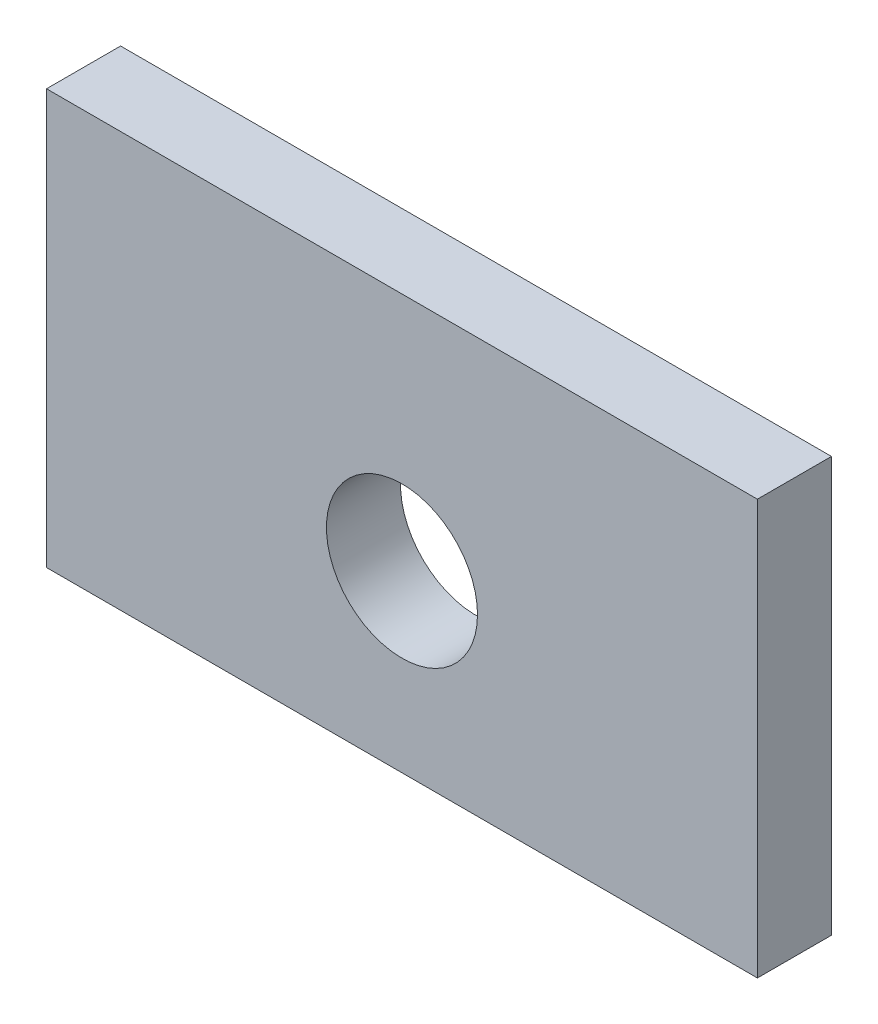
from build123d import *

# Parameters (mm, degrees)
SKETCH1_W           = 240
SKETCH1_H           = 140
SKETCH1_R           = 25.5
BOSS_EXTRUDE1_DEPTH = 25


with BuildPart() as part:
    # Sketch1 → Boss-Extrude1 (new body)
    with BuildSketch(Plane.XY):
        with Locations((120, 70)):
            Rectangle(SKETCH1_W, SKETCH1_H)
        with Locations((120, 59)):
            Circle(SKETCH1_R, mode=Mode.SUBTRACT)
    extrude(amount=BOSS_EXTRUDE1_DEPTH)


solid = part.part
